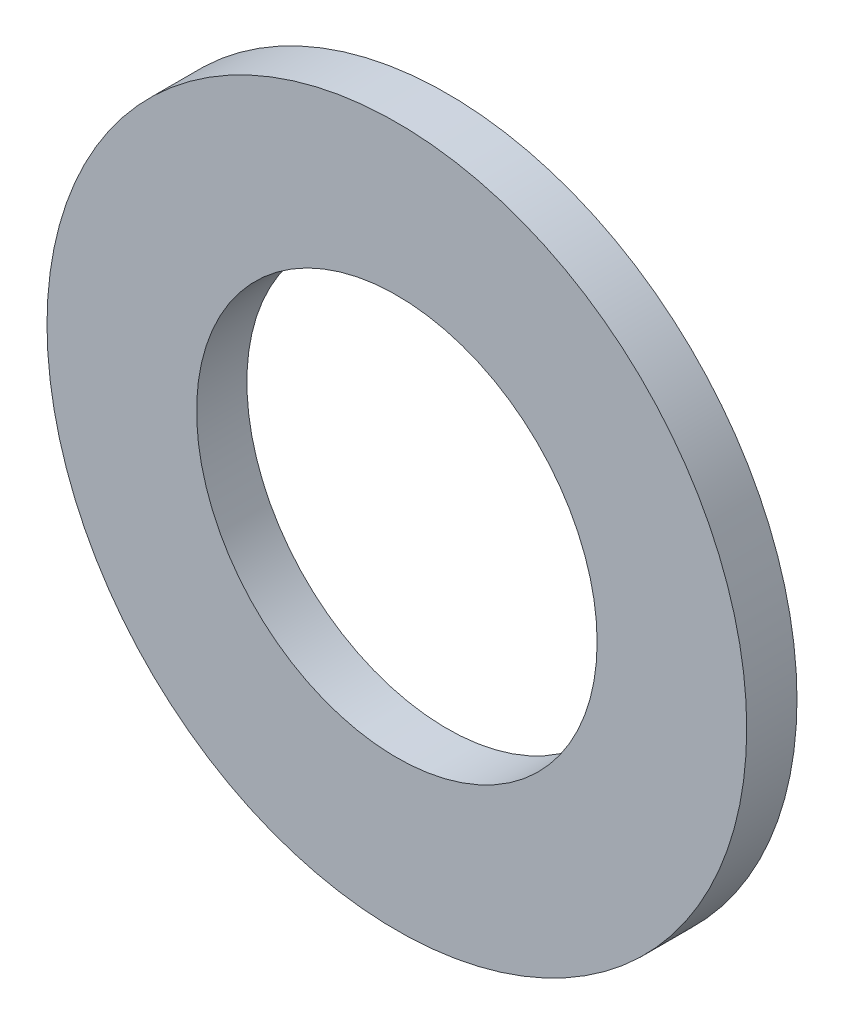
SolidWorks part; units mm, degrees
material "AISI 4130 Steel, normalized at 870C"
ref_plane "Front" through (0, 0, 0) normal (0, 0, 1) x (1, 0, 0)
ref_plane "Top" through (0, 0, 0) normal (0, 1, 0) x (1, 0, 0)
ref_plane "Right" through (0, 0, 0) normal (1, 0, 0) x (0, 0, -1)
sketch "Sketch1" plane through (0, 0, 0) normal (0, 0, 1) x (1, 0, 0)
  circle A0 centre (0, 0) radius 11.1379
  circle A1 centre (0, 0) radius 6.3754
  dimension "D1" = 12.7508
  dimension "D2" = 22.2758
extrude "Boss-Extrude1" add sketch "Sketch1" along normal blind 1.6002
